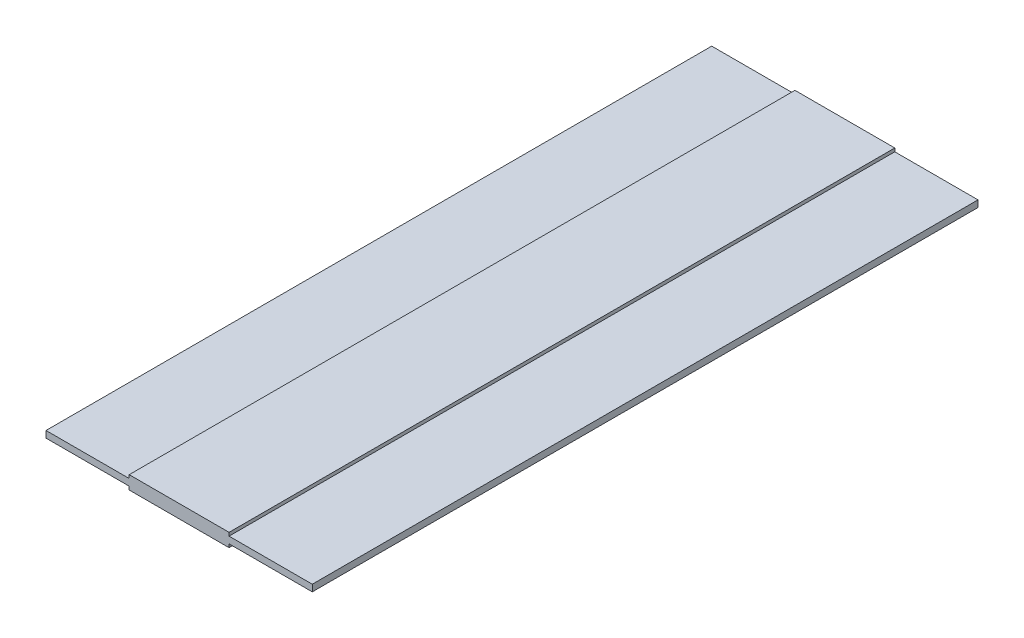
SolidWorks part; units mm, degrees
ref_plane "Front Plane" through (0, 0, 0) normal (0, 0, 1) x (1, 0, 0)
ref_plane "Top Plane" through (0, 0, 0) normal (0, 1, 0) x (1, 0, 0)
ref_plane "Right Plane" through (0, 0, 0) normal (1, 0, 0) x (0, 0, -1)
sketch "Sketch1" plane through (0, 0, 0) normal (0, 0, 1) x (1, 0, 0)
  line L1 (-100, 2.5) -> (100, 2.5)
  line L2 (-100, 2.5) -> (-100, -2.5)
  line L3 (-100, -2.5) -> (100, -2.5)
  line L4 (100, 2.5) -> (100, -2.5)
  line L5 (-100, 2.5) -> (100, -2.5) construction
  line L6 (-100, -2.5) -> (100, 2.5) construction
  point P0 (0, 0)
  dimension "D1" = 200
  dimension "D2" = 5
extrude "Boss-Extrude1" add sketch "Sketch1" along normal blind 500
sketch "Sketch2" plane through (0, 0, 500) normal (0, 0, 1) x (1, 0, 0)
  line L1 (-37.5, 5) -> (37.5, 5)
  line L2 (-37.5, 5) -> (-37.5, -5)
  line L3 (-37.5, -5) -> (37.5, -5)
  line L4 (37.5, 5) -> (37.5, -5)
  line L5 (-37.5, 5) -> (37.5, -5) construction
  line L6 (-37.5, -5) -> (37.5, 5) construction
  point P0 (0, 0)
  dimension "D1" = 10
  dimension "D2" = 75
extrude "Boss-Extrude2" add sketch "Sketch2" against normal blind 500
